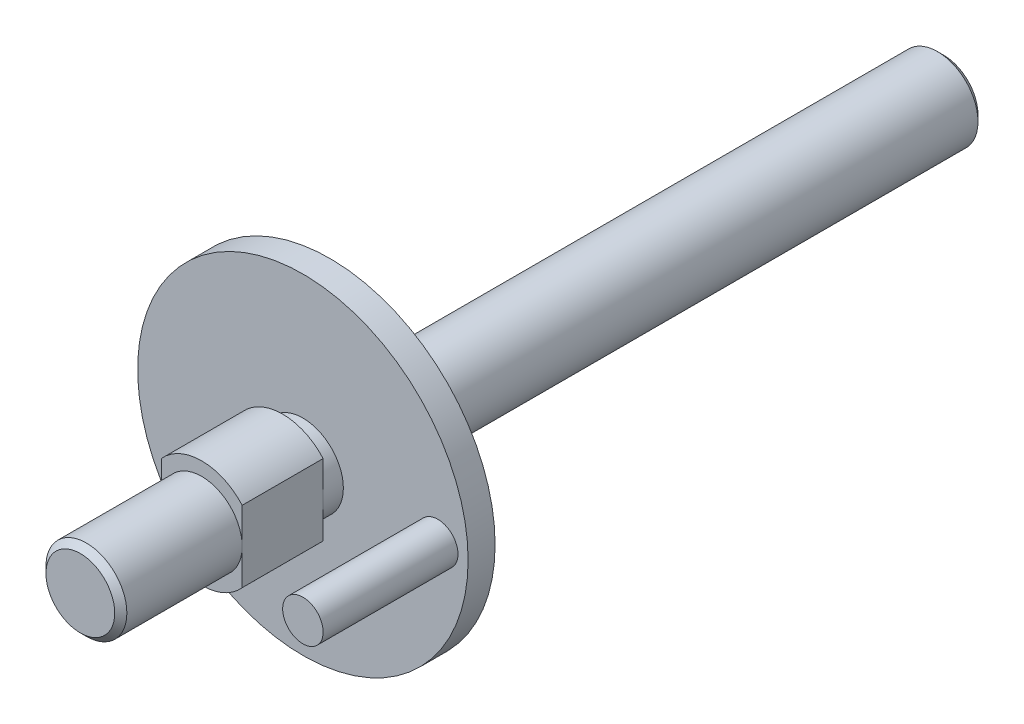
SolidWorks part; units mm, degrees
ref_plane "Front Plane" through (0, 0, 0) normal (0, 0, 1) x (1, 0, 0)
ref_plane "Top Plane" through (0, 0, 0) normal (0, 1, 0) x (1, 0, 0)
ref_plane "Right Plane" through (0, 0, 0) normal (1, 0, 0) x (0, 0, -1)
sketch "Sketch1" plane through (0, 0, 0) normal (0, 0, 1) x (1, 0, 0)
  circle A0 centre (0, 0) radius 6
extrude "Boss-Extrude1" add sketch "Sketch1" along normal blind 91
cosmetic thread "Cosmetic Thread1" parameters "D1"=70, "D2"=10.2
sketch "Sketch2" plane through (0, 0, 91) normal (0, 0, 1) x (1, 0, 0)
  circle A0 centre (0, 0) radius 24.5
extrude "Boss-Extrude2" add sketch "Sketch2" along normal blind 4
sketch "Sketch3" plane through (0, 0, 95) normal (0, 0, 1) x (1, 0, 0)
  circle A0 centre (0, 0) radius 6
extrude "Boss-Extrude3" add sketch "Sketch3" along normal blind 3
sketch "Sketch4" plane through (0, 0, 98) normal (0, 0, 1) x (1, 0, 0)
  line L1 (6, 5.2915) -> (6, -5.2915)
  line L3 (-6, 5.2915) -> (-6, -5.2915)
  arc A0 (-6, -5.2915) -> (6, -5.2915) centre (0, 0) ccw
  arc A1 (6, 5.2915) -> (-6, 5.2915) centre (0, 0) ccw
extrude "Boss-Extrude4" add sketch "Sketch4" along normal blind 12
sketch "Sketch5" plane through (0, 0, 110) normal (0, 0, 1) x (1, 0, 0)
  circle A0 centre (0, 0) radius 6 construction
  circle A1 centre (0, 0) radius 6
extrude "Boss-Extrude5" add sketch "Sketch5" along normal blind 18
cosmetic thread "Cosmetic Thread2" parameters "D1"=15, "D2"=10.2
chamfer "Chamfer1" distance 0.9 angle 45 2 edges at (6, 0, 0) (6, 0, 128)
sketch "Sketch6" plane through (0, 0, 95) normal (0, 0, 1) x (1, 0, 0)
  circle A0 centre (20, 0) radius 3
  dimension "D1" = 20
extrude "Boss-Extrude6" add sketch "Sketch6" along normal blind 20
sketch "Sketch7" plane through (0, 0, 0) normal (0, 1, 0) x (1, 0, 0)
  line L0 (-6, -95) -> (6, -95) construction
  line L1 (17, -95) -> (23, -95) construction
  point P0 (0, -95)
  point P1 (20, -95)
